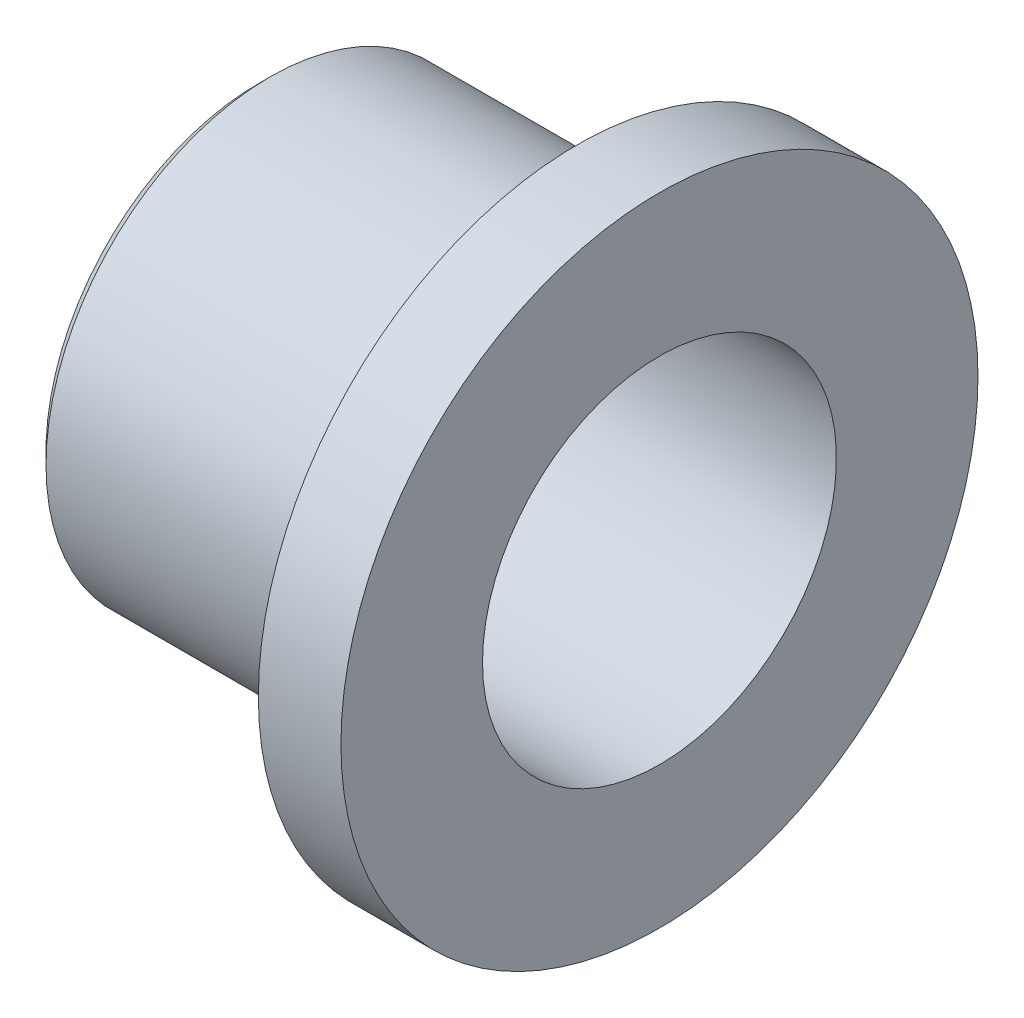
SolidWorks part; units mm, degrees
material "S45C"
ref_plane "Front Plane" through (0, 0, 0) normal (0, 0, 1) x (1, 0, 0)
ref_plane "Top Plane" through (0, 0, 0) normal (0, 1, 0) x (1, 0, 0)
ref_plane "Right Plane" through (0, 0, 0) normal (1, 0, 0) x (0, 0, -1)
sketch "Sketch1" plane through (0, 0, 0) normal (0, 0, 1) x (1, 0, 0)
  line L0 (0, 0) -> (76.6525, 0) construction
  line L1 (0, 15) -> (34, 15)
  line L2 (34, 15) -> (34, 27)
  line L3 (34, 27) -> (27, 27)
  line L4 (27, 27) -> (27, 19)
  line L5 (27, 19) -> (0, 19)
  line L6 (0, 19) -> (0, 15)
  dimension "D1" = 30
  dimension "D2" = 38
  dimension "D3" = 54
  dimension "D4" = 7
  dimension "D5" = 27
revolve "Revolve1" add sketch "Sketch1" angle 360 about L0
chamfer "Chamfer1" distance 1 angle 45 1 edges at (0, 0, 19)
